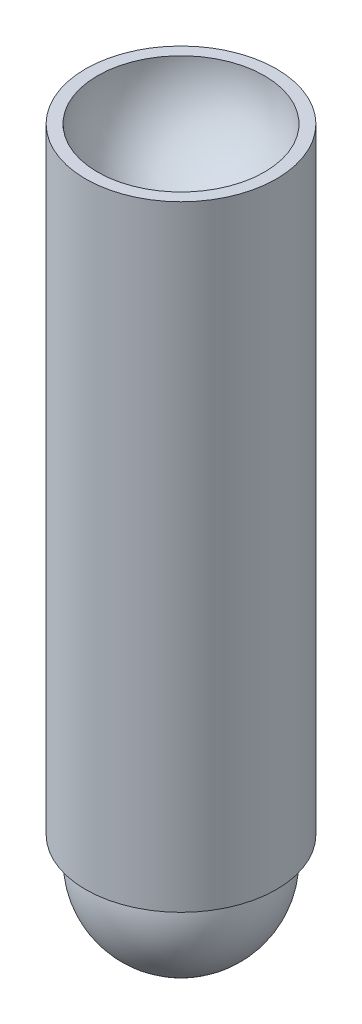
from build123d import *


with BuildPart() as part:
    # Sketch1 → Revolve2 (revolve)
    with BuildSketch(Plane.XY, mode=Mode.PRIVATE) as revolve2_sk:
        with BuildLine():
            Line((-2, 0), (-2, 53.291796068))
            ThreePointArc((-2, 53.291796068), (-5.61248608, 55.816699867), (-7, 60))
            Line((-7, 60), (-8, 60))
            Line((-8, 60), (-8, 8.392398037))
            Line((-8, 8.392398037), (-6.75, 8.392398037))
            ThreePointArc((-6.75, 8.392398037), (-6.244894811, 3.375866985), (-2.5, 0))
            Line((-2.5, 0), (-2, 0))
        make_face()
    revolve(revolve2_sk.sketch.rotate(Axis((0, 0, 0), (0, 1, 0)), 270), axis=Axis((0, 0, 0), (0, 1, 0)))


solid = part.part
